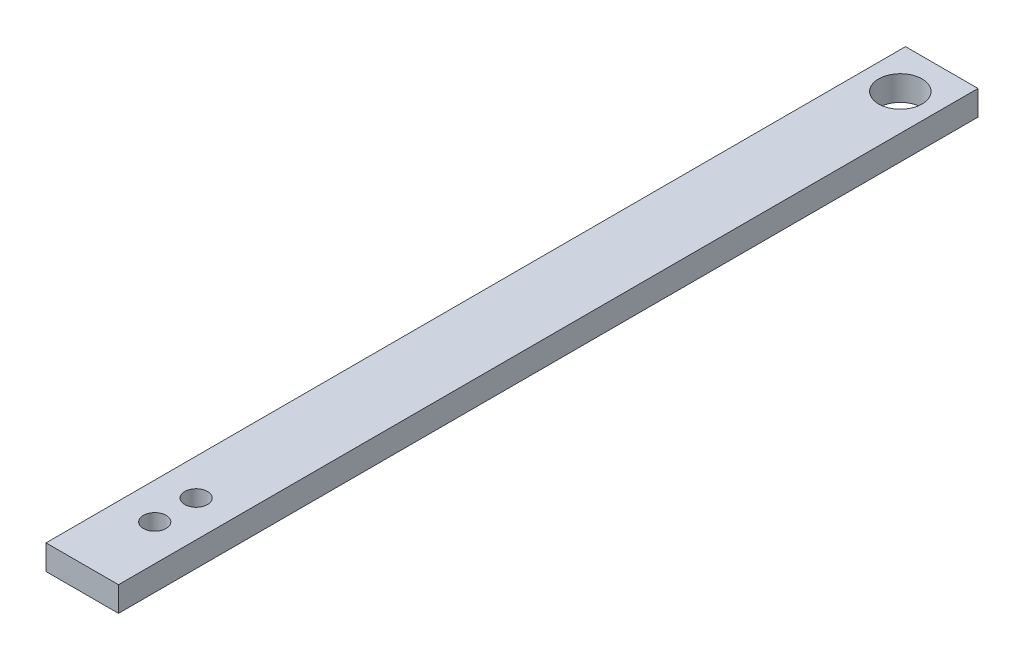
SolidWorks part; units mm, degrees
ref_plane "前视基准面" through (0, 0, 0) normal (0, 0, 1) x (1, 0, 0)
ref_plane "上视基准面" through (0, 0, 0) normal (0, 1, 0) x (1, 0, 0)
ref_plane "右视基准面" through (0, 0, 0) normal (1, 0, 0) x (0, 0, -1)
sketch "草图1" plane through (0, 0, 0) normal (0, 0, 1) x (1, 0, 0)
  line L1 (-17.5, -6) -> (17.5, -6)
  line L2 (-17.5, -6) -> (-17.5, 6)
  line L3 (-17.5, 6) -> (17.5, 6)
  line L4 (17.5, -6) -> (17.5, 6)
  line L5 (-17.5, -6) -> (17.5, 6) construction
  line L6 (-17.5, 6) -> (17.5, -6) construction
  point P0 (0, 0)
  dimension "D1" = 35
  dimension "D2" = 12
extrude "凸台-拉伸1" add sketch "草图1" along normal mid plane 415
sketch "草图2" plane through (0, 6, 0) normal (0, 1, 0) x (1, 0, 0)
  line L0 (0, 0) -> (0, -360.3152) construction
  line L1 (17.5, -207.5) -> (-17.5, -207.5) construction
  line L2 (0, -55) -> (0, 55) construction
  line L3 (17.5, 207.5) -> (-17.5, 207.5) construction
  circle A0 centre (0, 187.5) radius 10.5
  circle A1 centre (0, -152.5) radius 5.5
  circle A2 centre (0, -172.5) radius 5.5
  dimension "D1" = 21
  dimension "D3" = 11
  dimension "D4" = 11
  dimension "D2" = 20
  dimension "D5" = 35
  dimension "D6" = 20
extrude "切除-拉伸1" cut sketch "草图2" against normal up to surface (12 mm away) up to face at (0, -6, 0)
